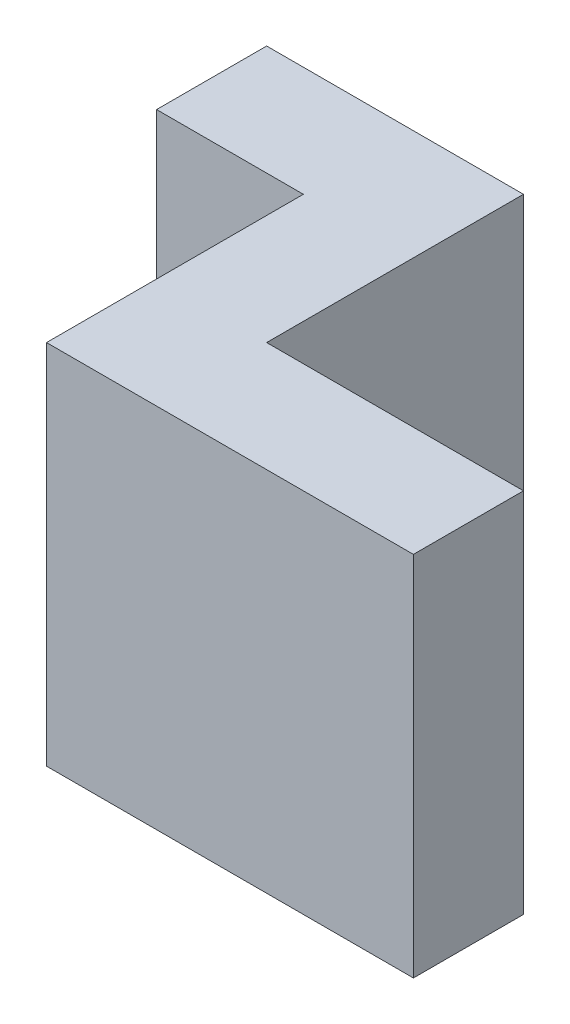
from build123d import *

# Parameters (mm, degrees)
BOSS_EXTRUDE1_DEPTH = 10


with BuildPart() as part:
    # Sketch1 → Boss-Extrude1 (new body)
    with BuildSketch(Plane(origin=(0, 0, 0), x_dir=(1, 0, 0), z_dir=(0, 1, 0))):
        Polygon((0, 0), (4, 0), (4, -7), (14, -7), (14, -4), (7, -4), (7, 3), (0, 3), align=None)
    extrude(amount=BOSS_EXTRUDE1_DEPTH)


solid = part.part
